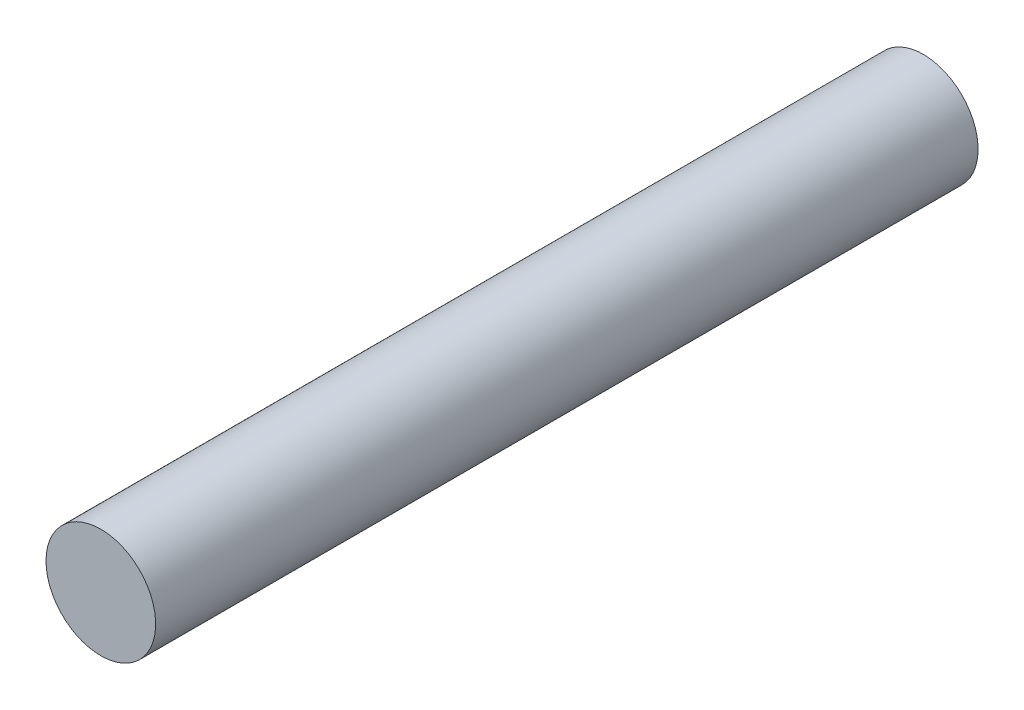
from build123d import *

# Parameters (mm, degrees)
SKETCH1_R           = 3
BOSS_EXTRUDE1_DEPTH = 22.5


with BuildPart() as part:
    # Sketch1 → Boss-Extrude1 (new, symmetric)
    with BuildSketch(Plane.XY):
        with Locations(Location((0, 0, 0), (0, 0, 180))):
            Circle(SKETCH1_R)
    extrude(amount=BOSS_EXTRUDE1_DEPTH, both=True)


solid = part.part
